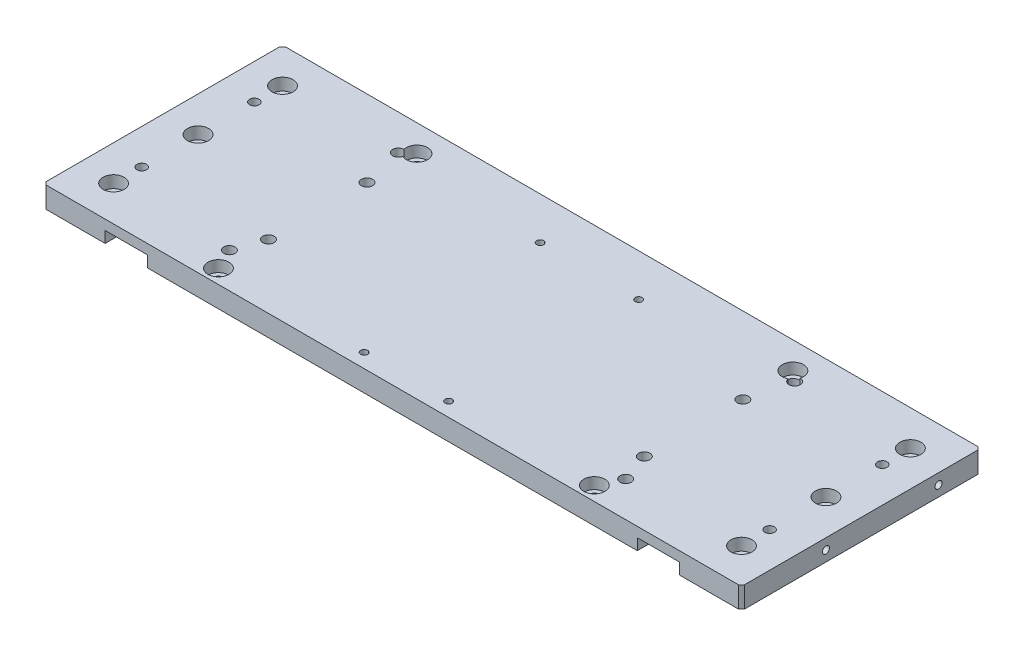
from build123d import *

# Parameters (mm, degrees)
SKETCH1_W                                           = 496
SKETCH1_H                                           = 170
BOSS_EXTRUDE1_DEPTH                                 = 15
CBORE_FOR_M8_HEX_SOCKET_HEAD_CAP_SCREW2_D           = 9
CBORE_FOR_M8_HEX_SOCKET_HEAD_CAP_SCREW2_CBORE_D     = 15
CBORE_FOR_M8_HEX_SOCKET_HEAD_CAP_SCREW2_CBORE_DEPTH = 8.6
SKETCH4_R                                           = 4
CUT_EXTRUDE1_DEPTH                                  = 263.59093663
SKETCH5_R                                           = 4
CUT_EXTRUDE2_DEPTH                                  = 263.59093663
CBORE_FOR_M8_HEX_SOCKET_HEAD_CAP_SCREW1_D           = 9
CBORE_FOR_M8_HEX_SOCKET_HEAD_CAP_SCREW1_CBORE_D     = 15
CBORE_FOR_M8_HEX_SOCKET_HEAD_CAP_SCREW1_CBORE_DEPTH = 8
M6_TAPPED_HOLE1_D                                   = 5
M6_TAPPED_HOLE1_DEPTH                               = 15
M6_TAPPED_HOLE1_TIP                                 = 1.502151548
M6_TAPPED_HOLE2_D                                   = 5
CHAMFER1_SIZE                                       = 2
M6_TAPPED_HOLE3_D                                   = 5
M6_TAPPED_HOLE4_D                                   = 5
M6_TAPPED_HOLE4_DEPTH                               = 15
M6_TAPPED_HOLE4_TIP                                 = 1.502151548
M8_TAPPED_HOLE1_D                                   = 6.8
SKETCH18_W                                          = 30
SKETCH18_H                                          = 170
CUT_EXTRUDE3_DEPTH                                  = 8


with BuildPart() as part:
    # Sketch1 → Boss-Extrude1 (new body)
    with BuildSketch(Plane(origin=(0, 0, 0), x_dir=(1, 0, 0), z_dir=(0, 1, 0))):
        Rectangle(SKETCH1_W, SKETCH1_H)
    extrude(amount=BOSS_EXTRUDE1_DEPTH)

    # CBORE for M8 Hex Socket Head Cap Screw2 (through all)
    with Locations(Plane(origin=(0, 15, 0), x_dir=(-1, 0, 0), z_dir=(0, 1, 0))):
        with Locations((223, -60), (223, 0), (223, 60)):
            cbore_for_m8_hex_socket_head_cap_screw2 = CounterBoreHole(CBORE_FOR_M8_HEX_SOCKET_HEAD_CAP_SCREW2_D / 2, CBORE_FOR_M8_HEX_SOCKET_HEAD_CAP_SCREW2_CBORE_D / 2, CBORE_FOR_M8_HEX_SOCKET_HEAD_CAP_SCREW2_CBORE_DEPTH)

    # Sketch4 → Cut-Extrude1 (cut, through all)
    with BuildSketch(Plane.XZ):
        with Locations(Location((140.75, 60, 0), (0, 0, 270))):
            Circle(SKETCH4_R)
        with Locations(Location((140.75, -60, 0), (0, 0, 270))):
            Circle(SKETCH4_R)
        with Locations(Location((-140.75, -60, 0), (0, 0, 270))):
            Circle(SKETCH4_R)
        with Locations(Location((-140.75, 60, 0), (0, 0, 270))):
            Circle(SKETCH4_R)
    extrude(amount=-CUT_EXTRUDE1_DEPTH, mode=Mode.SUBTRACT)

    # Sketch5 → Cut-Extrude2 (cut, through all)
    with BuildSketch(Plane.XZ):
        with Locations(Location((133.5, -30.5, 0), (0, 0, 270))):
            Circle(SKETCH5_R)
        with Locations(Location((133.5, 39.5, 0), (0, 0, 270))):
            Circle(SKETCH5_R)
        with Locations(Location((-133.5, 39.5, 0), (0, 0, 270))):
            Circle(SKETCH5_R)
        with Locations(Location((-133.5, -30.5, 0), (0, 0, 270))):
            Circle(SKETCH5_R)
    extrude(amount=-CUT_EXTRUDE2_DEPTH, mode=Mode.SUBTRACT)

    # CBORE for M8 Hex Socket Head Cap Screw1 (through all)
    with Locations(Plane(origin=(0, 15, 0), x_dir=(-1, 0, 0), z_dir=(0, 1, 0))):
        with Locations((133.5, -66), (-133.5, -66), (133.5, 75), (-133.5, 75)):
            CounterBoreHole(CBORE_FOR_M8_HEX_SOCKET_HEAD_CAP_SCREW1_D / 2, CBORE_FOR_M8_HEX_SOCKET_HEAD_CAP_SCREW1_CBORE_D / 2, CBORE_FOR_M8_HEX_SOCKET_HEAD_CAP_SCREW1_CBORE_DEPTH)

    # M6 Tapped Hole1
    with Locations(Plane(origin=(248, 0, 0), x_dir=(0, 0, -1), z_dir=(1, 0, 0))):
        with Locations((55, 7.5), (-25, 7.5)):
            Hole(M6_TAPPED_HOLE1_D / 2, depth=M6_TAPPED_HOLE1_DEPTH)
            with Locations((0, 0, -(M6_TAPPED_HOLE1_DEPTH + M6_TAPPED_HOLE1_TIP / 2))):  # 118° drill point
                Cone(0, M6_TAPPED_HOLE1_D / 2, M6_TAPPED_HOLE1_TIP, mode=Mode.SUBTRACT)

    # M6 Tapped Hole2 (through all)
    with Locations(Plane.XZ):
        with Locations((-35, -55), (35, -55)):
            Hole(M6_TAPPED_HOLE2_D / 2)

    # Chamfer1
    chamfer1_edges = [part.edges().sort_by_distance(p)[0] for p in [
        (248, 7.5, 85),
        (-248, 7.5, 85),
        (248, 7.5, -85),
        (-248, 7.5, -85),
    ]]
    chamfer(chamfer1_edges, length=CHAMFER1_SIZE)

    # M6 Tapped Hole3 (through all)
    with Locations(Plane.XZ):
        with Locations((-30, 75), (30, 75)):
            Hole(M6_TAPPED_HOLE3_D / 2)

    # M6 Tapped Hole4
    with Locations(Plane(origin=(0, 0, -85), x_dir=(-1, 0, 0), z_dir=(0, 0, -1))):
        with Locations((0, 7.5), (100, 7.5), (-100, 7.5)):
            Hole(M6_TAPPED_HOLE4_D / 2, depth=M6_TAPPED_HOLE4_DEPTH)
            with Locations((0, 0, -(M6_TAPPED_HOLE4_DEPTH + M6_TAPPED_HOLE4_TIP / 2))):  # 118° drill point
                Cone(0, M6_TAPPED_HOLE4_D / 2, M6_TAPPED_HOLE4_TIP, mode=Mode.SUBTRACT)

    # Mirror1: CBORE for M8 Hex Socket Head Cap Screw2 across plane
    add(cbore_for_m8_hex_socket_head_cap_screw2.mirror(Plane(origin=(0, 0, 0), x_dir=(0, 0, 1), z_dir=(1, 0, 0))), mode=Mode.SUBTRACT)

    # M8 Tapped Hole1 (through all)
    with Locations(Plane.XZ):
        with Locations((-223, 40), (-223, -40), (223, -40), (223, 40)):
            Hole(M8_TAPPED_HOLE1_D / 2)

    # Sketch18 → Cut-Extrude3 (cut)
    with BuildSketch(Plane.XZ):
        with Locations((-189, 0)):
            Rectangle(SKETCH18_W, SKETCH18_H)
        with Locations((189, 0)):
            Rectangle(SKETCH18_W, SKETCH18_H)
    extrude(amount=-CUT_EXTRUDE3_DEPTH, mode=Mode.SUBTRACT)


solid = part.part
